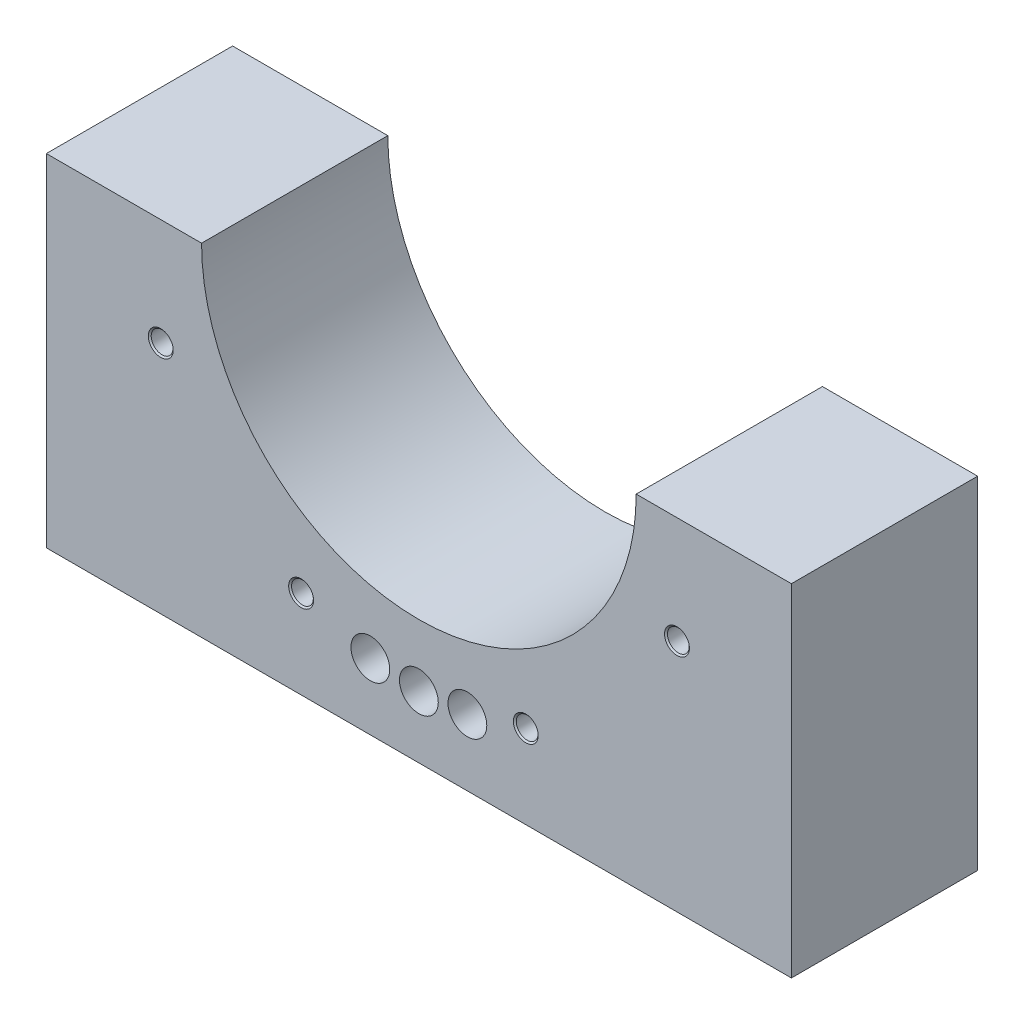
from build123d import *

# Parameters (mm, degrees)
SKETCH1_W                    = 480
SKETCH1_H                    = 220
BOSS_EXTRUDE1_DEPTH          = 120
CUT_EXTRUDE1_DEPTH           = 291
CUT_EXTRUDE1_DEPTH_BACK      = 291
SKETCH2_R                    = 140
CUT_EXTRUDE2_DEPTH           = 291
CUT_EXTRUDE2_DEPTH_BACK      = 291
SKETCH4_R                    = 12.5
M16_TAPPED_HOLE1_D           = 14
M16_TAPPED_HOLE1_DEPTH       = 32
M16_TAPPED_HOLE1_CSINK_D     = 16.05
M16_TAPPED_HOLE1_CSINK_ANGLE = 100
M16_TAPPED_HOLE1_TIP         = 4.206024333


with BuildPart() as part:
    # Sketch1 → Boss-Extrude1 (new body)
    with BuildSketch(Plane.XY):
        Rectangle(SKETCH1_W, SKETCH1_H)
    extrude(amount=BOSS_EXTRUDE1_DEPTH)

    # Sketch2 → Cut-Extrude1 (cut, two sides: drawn at the far end of the back side and taken through both)
    with BuildSketch(Plane.XY.offset(120).offset(-CUT_EXTRUDE1_DEPTH_BACK)):
        with Locations((0, 110)):
            Circle(SKETCH2_R)
    extrude(amount=CUT_EXTRUDE1_DEPTH + CUT_EXTRUDE1_DEPTH_BACK, mode=Mode.SUBTRACT)

    # Sketch4 → Cut-Extrude2 (cut, two sides: drawn at the far end of the back side and taken through both)
    with BuildSketch(Plane.XY.offset(120).offset(-CUT_EXTRUDE2_DEPTH_BACK)):
        with Locations((0, -70)):
            Circle(SKETCH4_R)
        with Locations((-31.25667198, -67.265395542)):
            Circle(SKETCH4_R)
        with Locations((31.25667198, -67.265395542)):
            Circle(SKETCH4_R)
    extrude(amount=CUT_EXTRUDE2_DEPTH + CUT_EXTRUDE2_DEPTH_BACK, mode=Mode.SUBTRACT)

    # M16 Tapped Hole1
    with Locations(Plane.XY.offset(120)):
        with Locations((-166.298315852, 41.116982174), (166.298315852, 41.116982174), (68.883017826, -56.298315852), (-75.868170831, -53.229962491)):
            CounterSinkHole(M16_TAPPED_HOLE1_D / 2, M16_TAPPED_HOLE1_CSINK_D / 2, depth=M16_TAPPED_HOLE1_DEPTH, counter_sink_angle=M16_TAPPED_HOLE1_CSINK_ANGLE)
            with Locations((0, 0, -(M16_TAPPED_HOLE1_DEPTH + M16_TAPPED_HOLE1_TIP / 2))):  # 118° drill point
                Cone(0, M16_TAPPED_HOLE1_D / 2, M16_TAPPED_HOLE1_TIP, mode=Mode.SUBTRACT)


solid = part.part
